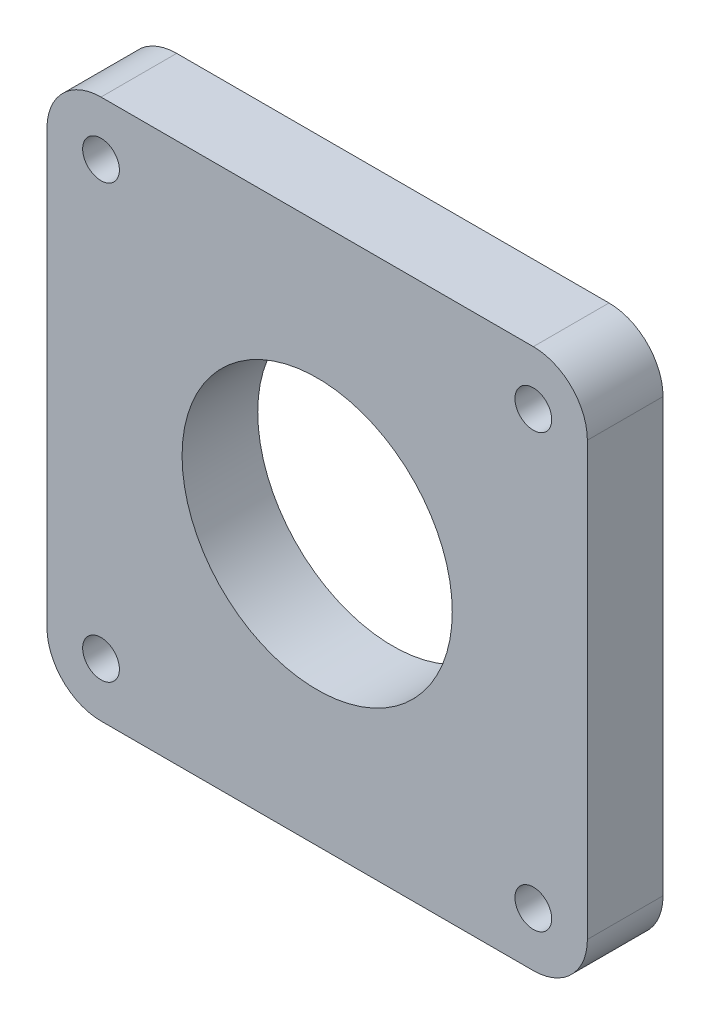
SolidWorks part; units mm, degrees
ref_plane "Front Plane" through (0, 0, 0) normal (0, 0, 1) x (1, 0, 0)
ref_plane "Top Plane" through (0, 0, 0) normal (0, 1, 0) x (1, 0, 0)
ref_plane "Right Plane" through (0, 0, 0) normal (1, 0, 0) x (0, 0, -1)
sketch "Sketch1" plane through (0, 0, 0) normal (0, 0, 1) x (1, 0, 0)
  line L1 (0, 0) -> (100, 0)
  line L2 (0, 0) -> (0, -100)
  line L3 (0, -100) -> (100, -100)
  line L4 (100, 0) -> (100, -100)
  dimension "D1" = 100
  dimension "D2" = 100
extrude "Boss-Extrude1" add sketch "Sketch1" along normal blind 14
sketch "Sketch2" plane through (0, 0, 14) normal (0, 0, 1) x (1, 0, 0)
  line L0 (0, -50) -> (50, -50) construction
  line L1 (0, 0) -> (0, -100) construction
  line L2 (50, 0) -> (50, -50) construction
  line L3 (100, 0) -> (0, 0) construction
  circle A0 centre (50, -50) radius 25
  dimension "D1" = 50
extrude "Cut-Extrude1" cut sketch "Sketch2" against normal through all
hole_wizard "M8 Tapped Hole1" positions "Sketch3" profile "Sketch4" tap size "M8" standard "GB" end condition through all
sketch "Sketch3" plane through (0, 0, 14) normal (0, 0, 1) x (1, 0, 0)
  line L1 (50, 0) -> (50, -100) construction
  line L2 (100, 0) -> (0, 0) construction
  line L3 (0, -100) -> (100, -100) construction
  line L5 (50, -50) -> (100, -50) construction
  line L6 (100, -100) -> (100, 0) construction
  point P0 (10, -10)
  point P2 (90, -10)
  point P4 (10, -90)
  point P6 (90, -90)
  dimension "D1" = 80
  dimension "D2" = 80
sketch "Sketch4" plane through (10, -10, 14) normal (1, 0, 0) x (0, -1, 0)
  line L0 (0, 0) -> (0, 14)
  line L1 (0, 14) -> (3.4, 14)
  line L2 (3.4, 14) -> (3.4, 0)
  line L5 (3.4, 0) -> (0, 0)
  line L11 (0, -6.35) -> (0, 107.95) construction
  dimension "通孔螺纹孔钻头直径" = 6.8
  dimension "通孔螺纹孔钻头深度" = 14
cosmetic thread "Hole thread1" parameters "D2"=8
cosmetic thread "Hole thread2" parameters "D2"=8
cosmetic thread "Hole thread3" parameters "D2"=8
cosmetic thread "Hole thread4" parameters "D2"=8
sketch "Sketch5" plane through (0, 0, 14) normal (0, 0, 1) x (1, 0, 0)
  circle A0 centre (50, -50) radius 30
  dimension "D1" = 60
extrude "Boss-Extrude2" [suppressed] add sketch "Sketch5" along normal blind 316
fillet "Fillet1" radius 10 4 edges at (0, -100, 7) (100, -100, 7) (100, 0, 7) (0, 0, 7)
